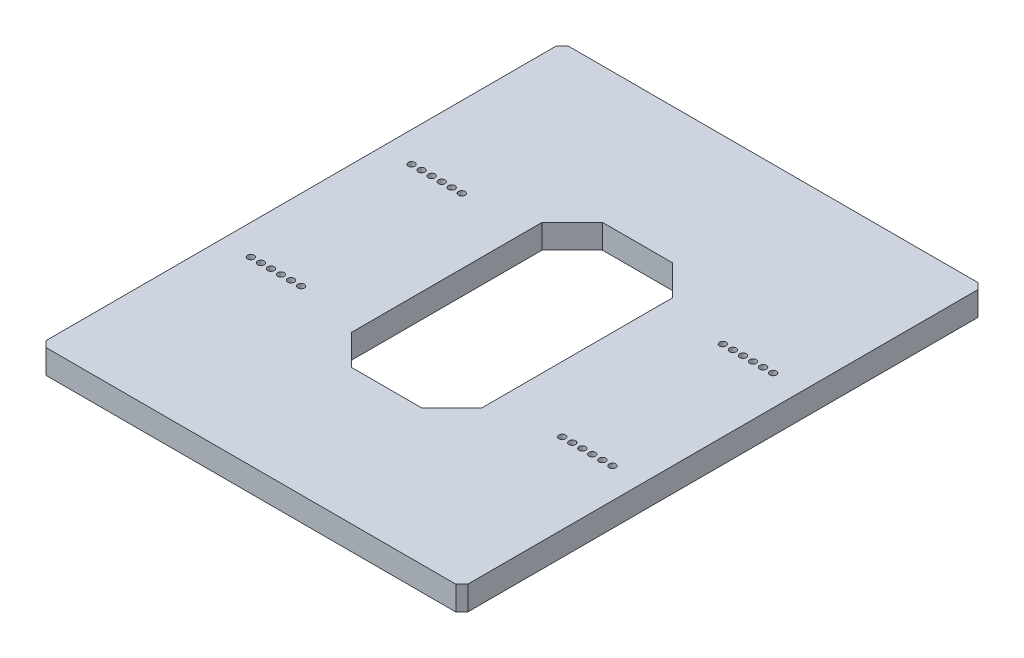
SolidWorks part; units mm, degrees
ref_plane "前视基准面" through (0, 0, 0) normal (0, 0, 1) x (1, 0, 0)
ref_plane "上视基准面" through (0, 0, 0) normal (0, 1, 0) x (1, 0, 0)
ref_plane "右视基准面" through (0, 0, 0) normal (1, 0, 0) x (0, 0, -1)
sketch "草图1" plane through (0, 0, 0) normal (0, 1, 0) x (1, 0, 0)
  line L1 (-105, -130) -> (105, -130)
  line L2 (-105, -130) -> (-105, 130)
  line L3 (-105, 130) -> (105, 130)
  line L4 (105, -130) -> (105, 130)
  line L5 (-105, -130) -> (105, 130) construction
  line L6 (-105, 130) -> (105, -130) construction
  point P0 (0, 0)
  dimension "D1" = 210
  dimension "D2" = 260
extrude "凸台-拉伸1" add sketch "草图1" along normal blind 12
hole_wizard "M4 螺纹孔1" positions "3D草图1" profile "草图2" tap size "M4" standard "GB" end condition up to next
sketch3d "3D草图1"
  line L0 (-105, 0, 0) -> (105, 0, 0) construction
  line L1 (-105, 0, -130) -> (-105, 0, 130) construction
  line L2 (105, 0, 130) -> (105, 0, -130) construction
  point P0 (-90, 0, -40)
  dimension "D1" = 40
  dimension "D2" = 15
sketch "草图2" plane through (-90, 0, -40) normal (1, 0, 0) x (0, 0, -1)
  line L0 (0, 0) -> (0, 12.001)
  line L1 (0, 12.001) -> (1.65, 12.001)
  line L2 (1.65, 12.001) -> (1.65, 0.375)
  line L3 (1.65, 0.375) -> (2.025, 0)
  line L5 (2.025, 0) -> (0, 0)
  line L6 (-1.65, 0.375) -> (-2.025, 0) construction
  line L11 (0, -6.35) -> (0, 107.95) construction
  dimension "通孔螺纹孔钻头直径" = 3.3
  dimension "通孔螺纹孔钻头深度" = 12.001
  dimension "近端锥形沉头孔直径" = 4.05
  dimension "近端锥形沉头孔角度" = 90
cosmetic thread "孔螺蚊线1" parameters "D2"=4
pattern_linear "阵列(线性)1" count 6 spacing 5 along (1, 0, 0) of "M4 螺纹孔1"
mirror "镜向1" about plane through (0, 0, 0) normal (1, 0, 0) of "阵列(线性)1", "M4 螺纹孔1"
mirror "镜向2" about plane through (0, 0, 0) normal (0, 0, 1) of "镜向1", "阵列(线性)1", "M4 螺纹孔1"
chamfer "倒角1" distance 3 angle 45 4 edges at (-105, 6, -130) (105, 6, -130) (-105, 6, 130) (105, 6, 130)
sketch "草图3" plane through (0, 0, 0) normal (0, -1, 0) x (1, 0, 0)
  line L1 (32.5, 62.5) -> (-32.5, 62.5)
  line L2 (32.5, 62.5) -> (32.5, -62.5)
  line L3 (32.5, -62.5) -> (-32.5, -62.5)
  line L4 (-32.5, 62.5) -> (-32.5, -62.5)
  line L5 (32.5, 62.5) -> (-32.5, -62.5) construction
  line L6 (32.5, -62.5) -> (-32.5, 62.5) construction
  point P0 (0, 0)
  dimension "D1" = 125
  dimension "D2" = 65
extrude "切除-拉伸1" cut sketch "草图3" against normal up to next
chamfer "倒角2" distance 15 angle 45 4 edges at (32.5, 6, 62.5) (-32.5, 6, 62.5) (-32.5, 6, -62.5) (32.5, 6, -62.5)
